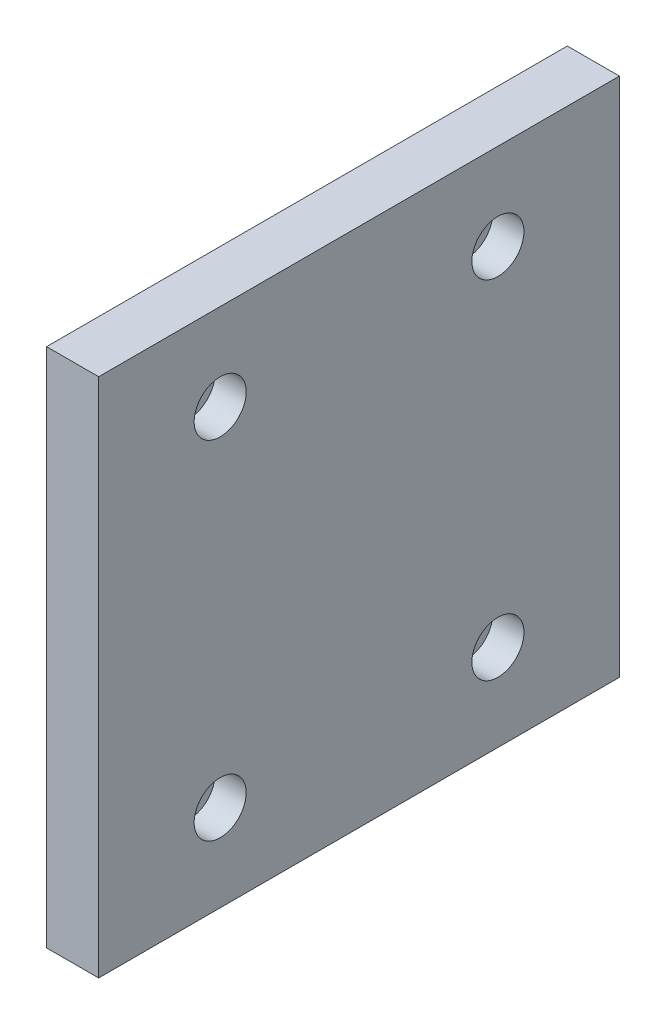
SolidWorks part; units mm, degrees
ref_plane "前视基准面" through (0, 0, 0) normal (0, 0, 1) x (1, 0, 0)
ref_plane "上视基准面" through (0, 0, 0) normal (0, 1, 0) x (1, 0, 0)
ref_plane "右视基准面" through (0, 0, 0) normal (1, 0, 0) x (0, 0, -1)
sketch "草图1" plane through (0, 0, 0) normal (1, 0, 0) x (0, 0, -1)
  line L1 (-75, 75) -> (75, 75)
  line L2 (-75, 75) -> (-75, -75)
  line L3 (-75, -75) -> (75, -75)
  line L4 (75, 75) -> (75, -75)
  line L5 (-75, 75) -> (75, -75) construction
  line L6 (-75, -75) -> (75, 75) construction
  point P0 (0, 0)
  dimension "D1" = 150
  dimension "D2" = 150
extrude "凸台-拉伸1" add sketch "草图1" along normal blind 15
hole_wizard "打孔尺寸(%根据)内六角圆柱头螺钉的类型1" positions "草图2" profile "草图3" counterbore size "M8" standard "GB" end condition through all
sketch "草图2" plane through (15, 0, 0) normal (1, 0, 0) x (0, 0, -1)
  line L0 (0, 48.4785) -> (0, 0) construction
  line L1 (0, 0) -> (86.8968, 0) construction
  point P0 (-40, 50)
  point P2 (40, 50)
  point P4 (-40, -50)
  point P6 (40, -50)
  dimension "D1" = 80
  dimension "D2" = 100
sketch "草图3" plane through (15, 50, 40) normal (0, 1, 0) x (0, 0, -1)
  line L0 (0, 0) -> (0, 15)
  line L1 (0, 15) -> (4.5, 15)
  line L3 (4.5, 15) -> (4.5, 9)
  line L4 (4.5, 9) -> (7.5, 9)
  line L5 (7.5, 9) -> (7.5, 0)
  line L7 (7.5, 0) -> (0, 0)
  line L11 (0, -6.35) -> (0, 107.95) construction
  dimension "通孔孔直径" = 9
  dimension "通孔孔深度" = 15
  dimension "柱形沉头孔直径" = 15
  dimension "柱形沉头孔深度" = 9
